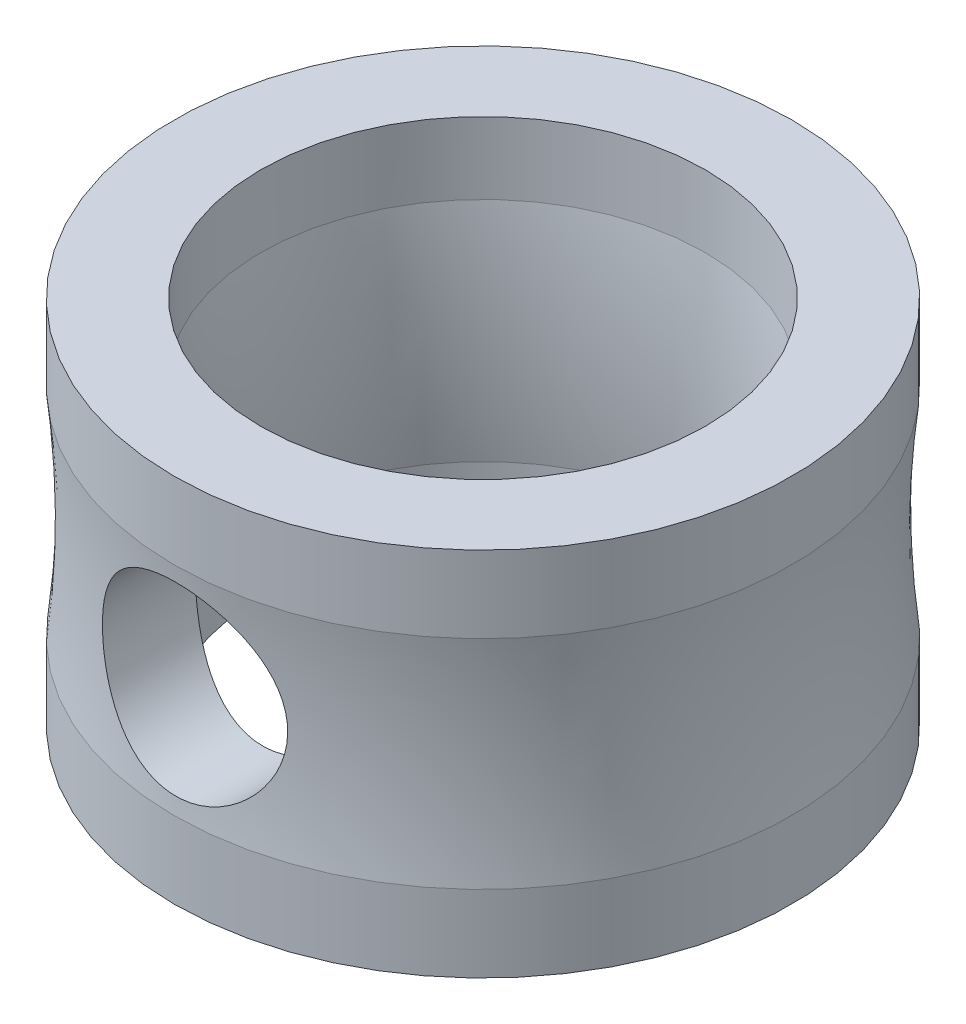
SolidWorks part; units mm, degrees
ref_plane "Front Plane" through (0, 0, 0) normal (0, 0, 1) x (1, 0, 0)
ref_plane "Top Plane" through (0, 0, 0) normal (0, 1, 0) x (1, 0, 0)
ref_plane "Right Plane" through (0, 0, 0) normal (1, 0, 0) x (0, 0, -1)
sketch "Sketch1" plane through (0, 0, 0) normal (0, 0, 1) x (1, 0, 0)
  line L0 (0, 0) -> (0, 300)
  line L1 (0, 300) -> (250, 300)
  line L2 (250, 300) -> (250, 237.8905)
  line L3 (0, 0) -> (250, 0)
  line L4 (250, 0) -> (250, 62.1095)
  line L5 (0, 150) -> (384.9315, 150) construction
  arc A1 (250, 237.8905) -> (250, 62.1095) centre (1000, 150) ccw
  dimension "D1" = 300
  dimension "D2" = 250
  dimension "D4" = 1000
revolve "Revolve1" add sketch "Sketch1" angle 360 about L0
shell "Shell1" thickness 70
sketch "Sketch2" plane through (0, 0, 0) normal (0, 0, 1) x (1, 0, 0)
  circle A0 centre (0, 150) radius 75
  dimension "D1" = 150
  dimension "D2" = 150
extrude "Cut-Extrude1" cut sketch "Sketch2" along normal blind 689
